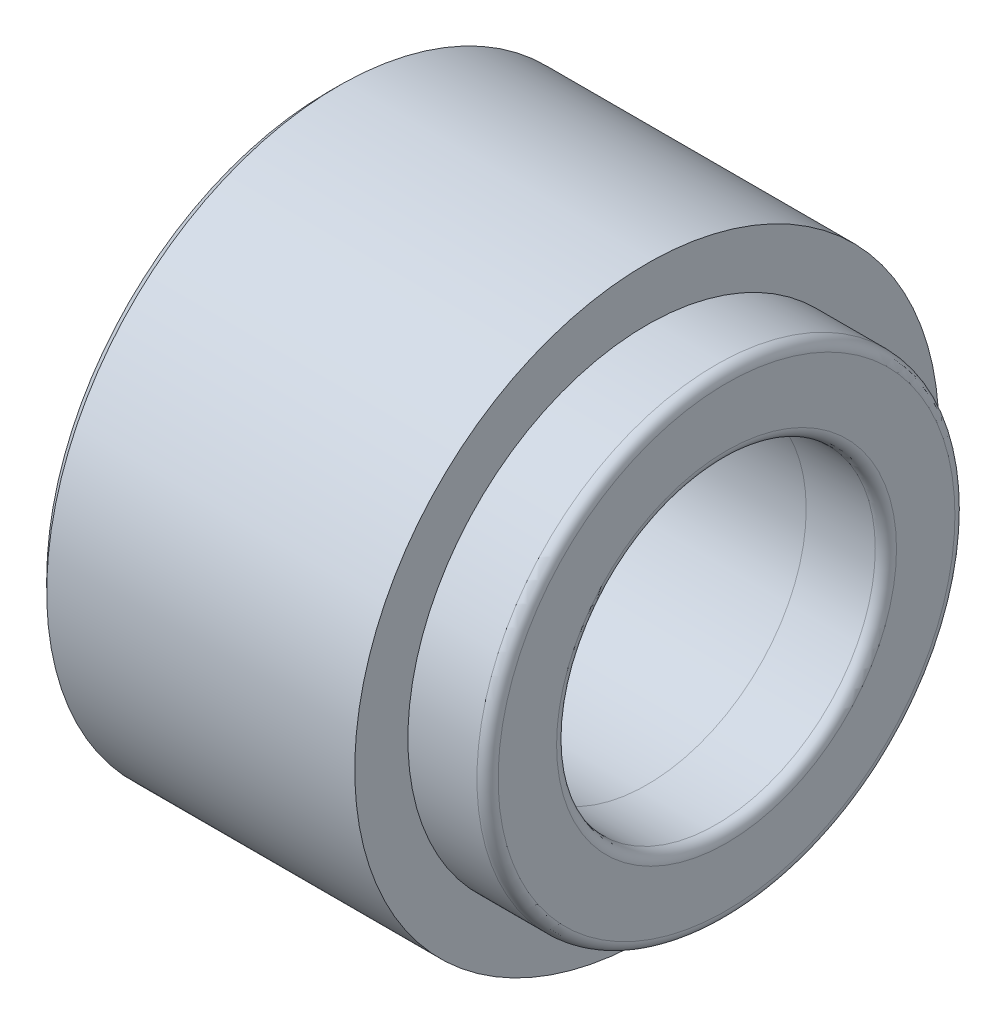
SolidWorks part; units mm, degrees
ref_plane "前视" through (0, 0, 0) normal (0, 0, 1) x (1, 0, 0)
ref_plane "上视" through (0, 0, 0) normal (0, 1, 0) x (1, 0, 0)
ref_plane "右视" through (0, 0, 0) normal (1, 0, 0) x (0, 0, -1)
sketch "草图1" plane through (0, 0, 0) normal (1, 0, 0) x (0, 0, -1)
  circle A0 centre (0, 0) radius 5.5
  circle A1 centre (0, 0) radius 3
extrude "凸台-拉伸1" add sketch "草图1" along normal blind 6
sketch "草图3" plane through (6, 0, 0) normal (1, 0, 0) x (0, 0, -1)
  circle A0 centre (0, 0) radius 3
  circle A1 centre (0, 0) radius 4.5
extrude "凸台-拉伸2" add sketch "草图3" along normal blind 1.5 separate body
fillet "圆角1" radius 0.2 2 edges at (7.5, 0, -4.5) (7.5, 0, -3)
chamfer "倒角1" distance 0.2 angle 45 2 edges at (0, 0, -3) (0, 0, -5.5)
